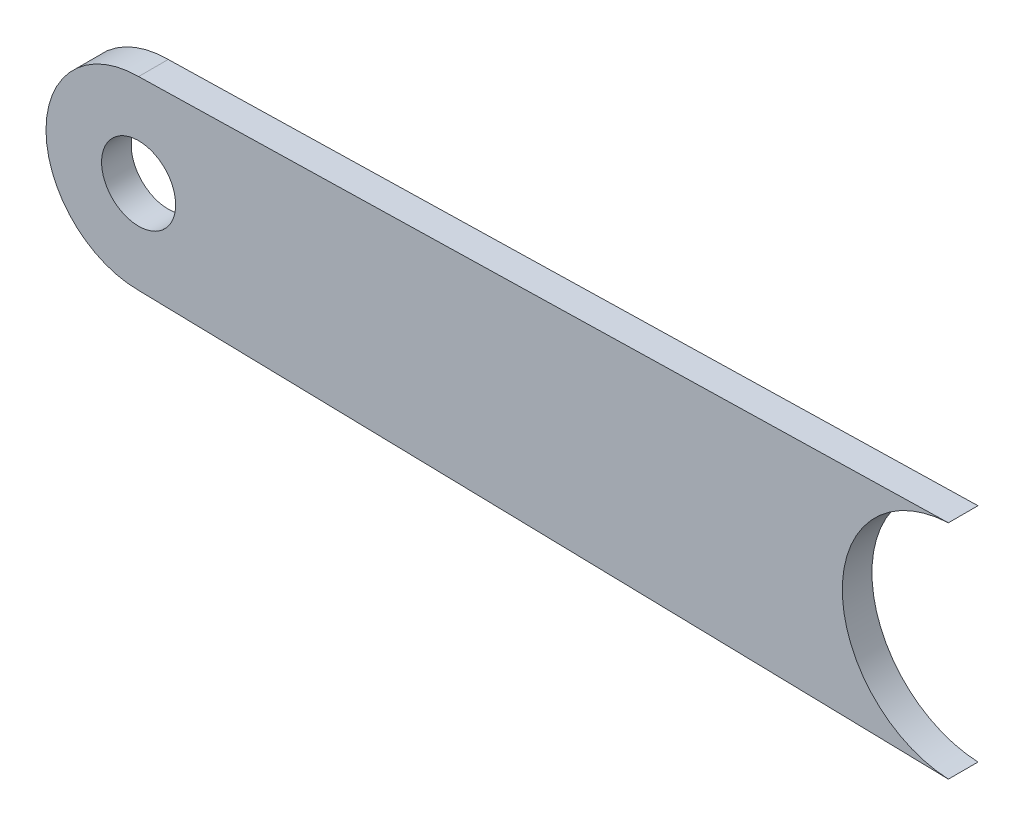
SolidWorks part; units mm, degrees
ref_plane "前视基准面" through (0, 0, 0) normal (0, 0, 1) x (1, 0, 0)
ref_plane "上视基准面" through (0, 0, 0) normal (0, 1, 0) x (1, 0, 0)
ref_plane "右视基准面" through (0, 0, 0) normal (1, 0, 0) x (0, 0, -1)
sketch "草图1" plane through (0, 0, 0) normal (0, 0, 1) x (1, 0, 0)
  line L0 (0, 25) -> (220, 30)
  line L3 (220, -30) -> (0, -25)
  arc A0 (0, 25) -> (0, -25) centre (0, 0) ccw
  arc A2 (220, 30) -> (220, -30) centre (220, 0) ccw
extrude "凸台-拉伸1" add sketch "草图1" along normal blind 8 contours A2 L0 A0 L3
sketch "草图2" plane through (0, 0, 8) normal (0, 0, 1) x (1, 0, 0)
  circle A0 centre (0, 0) radius 10
extrude "切除-拉伸1" cut sketch "草图2" against normal blind 8
